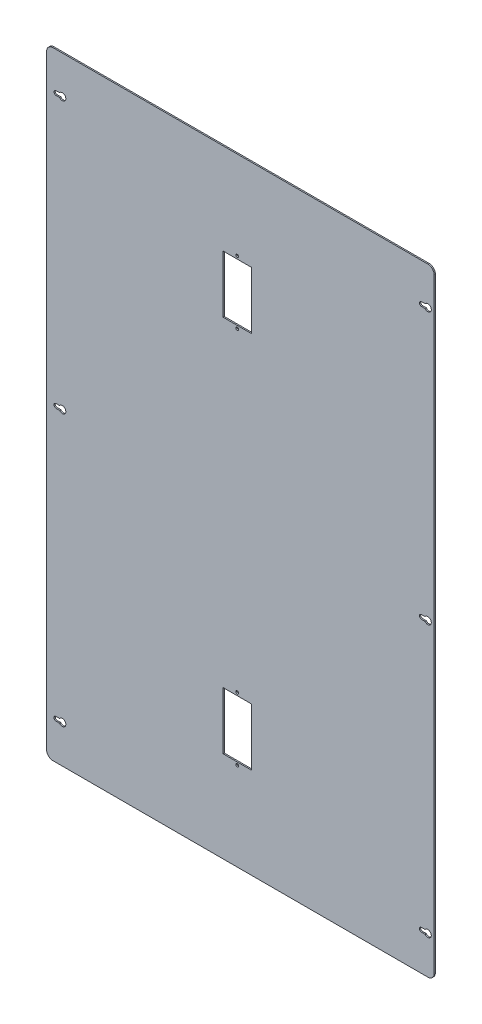
from build123d import *

# Parameters (mm, degrees)
SKETCH1_W            = 615
SKETCH1_H            = 980
BOSS_EXTRUDE1_DEPTH  = 2
SKETCH7_W            = 45
SKETCH7_H            = 91
CUT_EXTRUDE4_DEPTH   = 579.498271389
SKETCH8_R            = 2.25
CUT_EXTRUDE5_DEPTH   = 579.498271389
FILLET3_R            = 10
CUT_EXTRUDE6_DEPTH   = 10
LPATTERN1_COUNT      = 3
LPATTERN1_PITCH      = 430
LPATTERN1_COUNT_DIR2 = 2
LPATTERN1_PITCH_DIR2 = 580


with BuildPart() as part:
    # Sketch1 → Boss-Extrude1 (new body)
    with BuildSketch(Plane.XY):
        Rectangle(SKETCH1_W, SKETCH1_H)
    extrude(amount=BOSS_EXTRUDE1_DEPTH)

    # Sketch7 → Cut-Extrude4 (cut, through all)
    with BuildSketch(Plane(origin=(0, 0, 0), x_dir=(-1, 0, 0), z_dir=(0, 0, -1))):
        with Locations((5, 300)):
            Rectangle(SKETCH7_W, SKETCH7_H)
        with Locations((5, -300)):
            Rectangle(SKETCH7_W, SKETCH7_H)
    extrude(amount=-CUT_EXTRUDE4_DEPTH, mode=Mode.SUBTRACT)

    # Sketch8 → Cut-Extrude5 (cut, through all)
    with BuildSketch(Plane(origin=(0, 0, 0), x_dir=(-1, 0, 0), z_dir=(0, 0, -1))):
        with Locations((5, 350)):
            Circle(SKETCH8_R)
        with Locations((5, 250)):
            Circle(SKETCH8_R)
        with Locations((5, -250)):
            Circle(SKETCH8_R)
        with Locations((5, -350)):
            Circle(SKETCH8_R)
    extrude(amount=-CUT_EXTRUDE5_DEPTH, mode=Mode.SUBTRACT)

    # Fillet3
    fillet3_edges = [part.edges().sort_by_distance(p)[0] for p in [
        (307.5, -490, 1),
        (-307.5, -490, 1),
        (-307.5, 490, 1),
        (307.5, 490, 1),
    ]]
    fillet(fillet3_edges, radius=FILLET3_R)

    # Sketch10 → Cut-Extrude6 (cut)
    with BuildSketch(Plane(origin=(0, 0, 0), x_dir=(-1, 0, 0), z_dir=(0, 0, -1))):
        with BuildLine():
            Line((292.5, 433.3), (286.9, 433.3))
            ThreePointArc((286.9, 433.3), (277, 430), (286.9, 426.7))
            Line((286.9, 426.7), (292.5, 426.7))
            ThreePointArc((292.5, 426.7), (295.8, 430), (292.5, 433.3))
        make_face()
    cut_extrude6 = extrude(amount=-CUT_EXTRUDE6_DEPTH, mode=Mode.SUBTRACT)

    # LPattern1: Cut-Extrude6 3 × 2
    with Locations(*[(j * LPATTERN1_PITCH_DIR2, -i * LPATTERN1_PITCH, 0) for i in range(LPATTERN1_COUNT) for j in range(LPATTERN1_COUNT_DIR2) if (i, j) != (0, 0)]):
        add(cut_extrude6, mode=Mode.SUBTRACT)


solid = part.part
